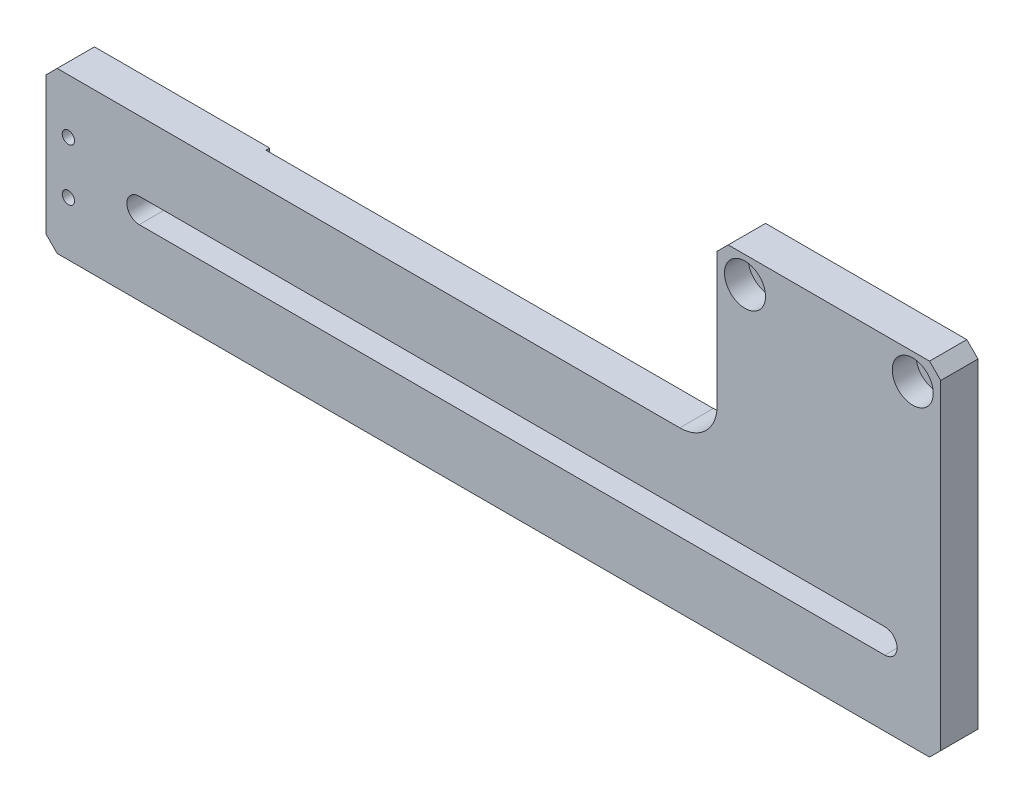
from build123d import *

# Parameters (mm, degrees)
SKETCH1_W                                           = 240
SKETCH1_H                                           = 92
BOSS_EXTRUDE1_DEPTH                                 = 10
CUT_EXTRUDE1_DEPTH                                  = 10
SKETCH3_W                                           = 180
SKETCH3_H                                           = 49
CUT_EXTRUDE2_DEPTH                                  = 10
FILLET1_R                                           = 10
CHAMFER1_SIZE                                       = 3
M4_TAPPED_HOLE1_D                                   = 3.3
M4_TAPPED_HOLE1_DEPTH                               = 11.5
M4_TAPPED_HOLE1_TIP                                 = 0.991420021
CBORE_FOR_M6_HEX_SOCKET_HEAD_CAP_SCREW1_D           = 6.4
CBORE_FOR_M6_HEX_SOCKET_HEAD_CAP_SCREW1_CBORE_D     = 11
CBORE_FOR_M6_HEX_SOCKET_HEAD_CAP_SCREW1_CBORE_DEPTH = 6.4
SKETCH8_W                                           = 130
SKETCH8_H                                           = 89
CUT_EXTRUDE3_DEPTH                                  = 1


with BuildPart() as part:
    # Sketch1 → Boss-Extrude1 (new body)
    with BuildSketch(Plane.XY):
        Rectangle(SKETCH1_W, SKETCH1_H)
    extrude(amount=BOSS_EXTRUDE1_DEPTH)

    # Sketch2 → Cut-Extrude1 (cut)
    with BuildSketch(Plane.XY.offset(10)):
        with BuildLine():
            Line((-95, -21.7), (105, -21.7))
            ThreePointArc((105, -21.7), (108.3, -25), (105, -28.3))
            Line((105, -28.3), (-95, -28.3))
            ThreePointArc((-95, -28.3), (-98.3, -25), (-95, -21.7))
        make_face()
    extrude(amount=-CUT_EXTRUDE1_DEPTH, mode=Mode.SUBTRACT)

    # Sketch3 → Cut-Extrude2 (cut)
    with BuildSketch(Plane.XY.offset(10)):
        with Locations((-30, 21.5)):
            Rectangle(SKETCH3_W, SKETCH3_H)
    extrude(amount=-CUT_EXTRUDE2_DEPTH, mode=Mode.SUBTRACT)

    # Fillet1
    fillet1_edges = [part.edges().sort_by_distance(p)[0] for p in [
        (60, -3, 5),
    ]]
    fillet(fillet1_edges, radius=FILLET1_R)

    # Chamfer1
    chamfer1_edges = [part.edges().sort_by_distance(p)[0] for p in [
        (-120, -3, 5),
        (60, 46, 5),
        (120, -46, 5),
        (-120, -46, 5),
        (120, 46, 5),
    ]]
    chamfer(chamfer1_edges, length=CHAMFER1_SIZE)

    # M4 Tapped Hole1
    with Locations(Plane.XY.offset(10)):
        with Locations((-114, -17.5), (-114, -31.5)):
            Hole(M4_TAPPED_HOLE1_D / 2, depth=M4_TAPPED_HOLE1_DEPTH)
            with Locations((0, 0, -(M4_TAPPED_HOLE1_DEPTH + M4_TAPPED_HOLE1_TIP / 2))):  # 118° drill point
                Cone(0, M4_TAPPED_HOLE1_D / 2, M4_TAPPED_HOLE1_TIP, mode=Mode.SUBTRACT)

    # CBORE for M6 Hex Socket Head Cap Screw1 (through all)
    with Locations(Plane.XY.offset(10)):
        with Locations((67.5, 39), (112.5, 39)):
            CounterBoreHole(CBORE_FOR_M6_HEX_SOCKET_HEAD_CAP_SCREW1_D / 2, CBORE_FOR_M6_HEX_SOCKET_HEAD_CAP_SCREW1_CBORE_D / 2, CBORE_FOR_M6_HEX_SOCKET_HEAD_CAP_SCREW1_CBORE_DEPTH)

    # Sketch8 → Cut-Extrude3 (cut)
    with BuildSketch(Plane(origin=(0, 0, 0), x_dir=(-1, 0, 0), z_dir=(0, 0, -1))):
        with Locations((5, -1.5)):
            Rectangle(SKETCH8_W, SKETCH8_H)
    extrude(amount=-CUT_EXTRUDE3_DEPTH, mode=Mode.SUBTRACT)


solid = part.part
